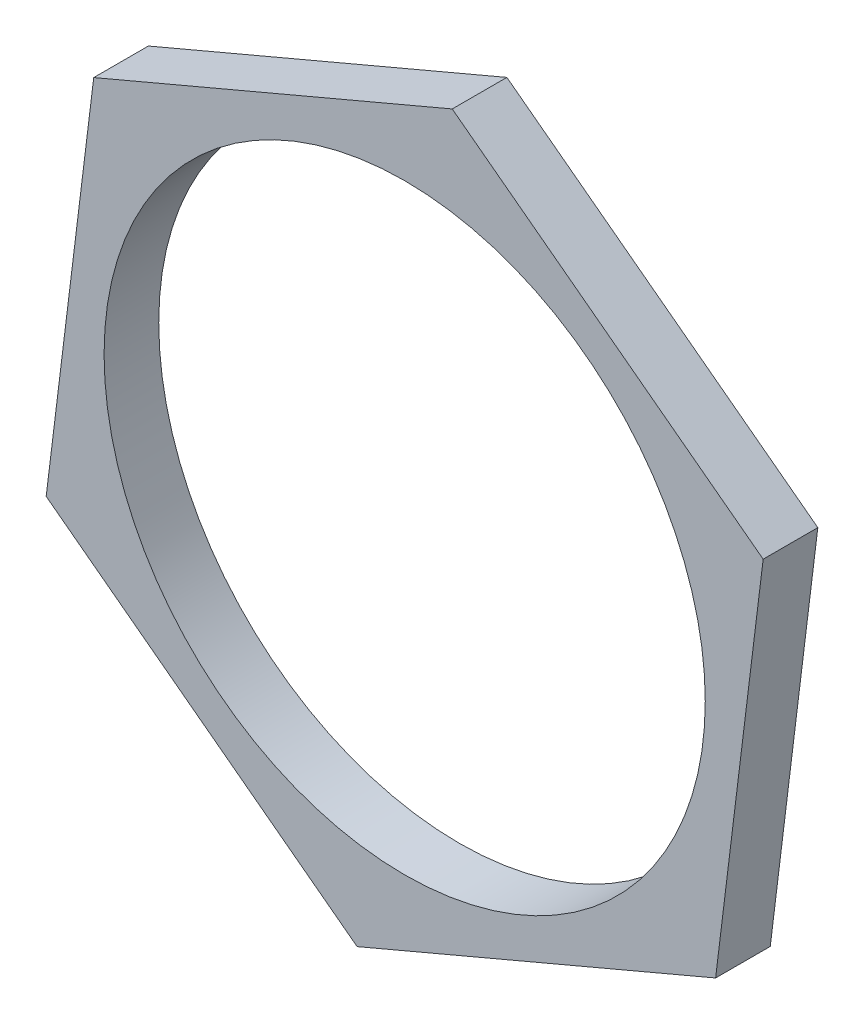
from build123d import *

# Parameters (mm, degrees)
SKETCH_1_R      = 11
EXTRUDE_1_DEPTH = 2


with BuildPart() as part:
    # 草图1 → 凸台-拉伸1 (new body)
    with BuildSketch(Plane.XY):
        Polygon((9.893192504, 17.474140349), (11.633566446, 31.61746381), (0.255276005, 40.196333587), (-12.863388378, 34.631879902), (-14.60376232, 20.48855644), (-3.225471879, 11.909686664), align=None)
        with Locations((-1.485097937, 26.053010125)):
            Circle(SKETCH_1_R, mode=Mode.SUBTRACT)
    extrude(amount=EXTRUDE_1_DEPTH)


solid = part.part
